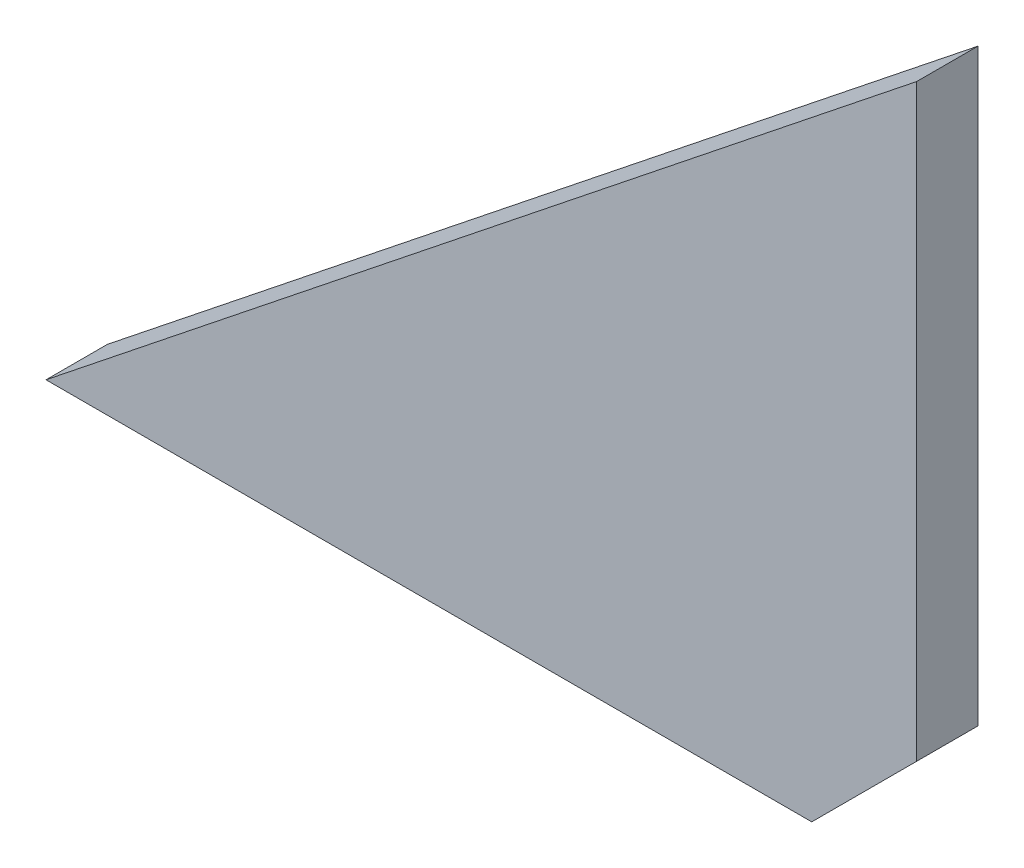
SolidWorks part; units mm, degrees
ref_plane "前视基准面" through (0, 0, 0) normal (0, 0, 1) x (1, 0, 0)
ref_plane "上视基准面" through (0, 0, 0) normal (0, 1, 0) x (1, 0, 0)
ref_plane "右视基准面" through (0, 0, 0) normal (1, 0, 0) x (0, 0, -1)
sketch "草图1" plane through (0, 0, 0) normal (0, 0, 1) x (1, 0, 0)
  line L0 (-5, 0) -> (-5, -47.9289)
  line L1 (-5, -47.9289) -> (-43.5355, -86.4645)
  line L2 (-43.5355, -86.4645) -> (-113.5355, -86.4645)
  line L3 (-113.5355, -86.4645) -> (-5, 0)
extrude "凸台-拉伸1" add sketch "草图1" along normal blind 5
sketch "草图2" plane through (0, 0, 5) normal (0, 0, 1) x (1, 0, 0)
  line L0 (-113.5355, -86.4645) -> (-113.5355, -56.4645)
  line L1 (-113.5355, -56.4645) -> (-13.5355, -56.4645)
  line L2 (-43.5355, -86.4645) -> (-5, -47.9289) construction
  line L3 (-13.5355, -56.4645) -> (-13.5355, -86.4645)
  line L4 (-13.5355, -86.4645) -> (-113.5355, -86.4645)
extrude "切除-拉伸1" cut sketch "草图2" against normal blind 360
